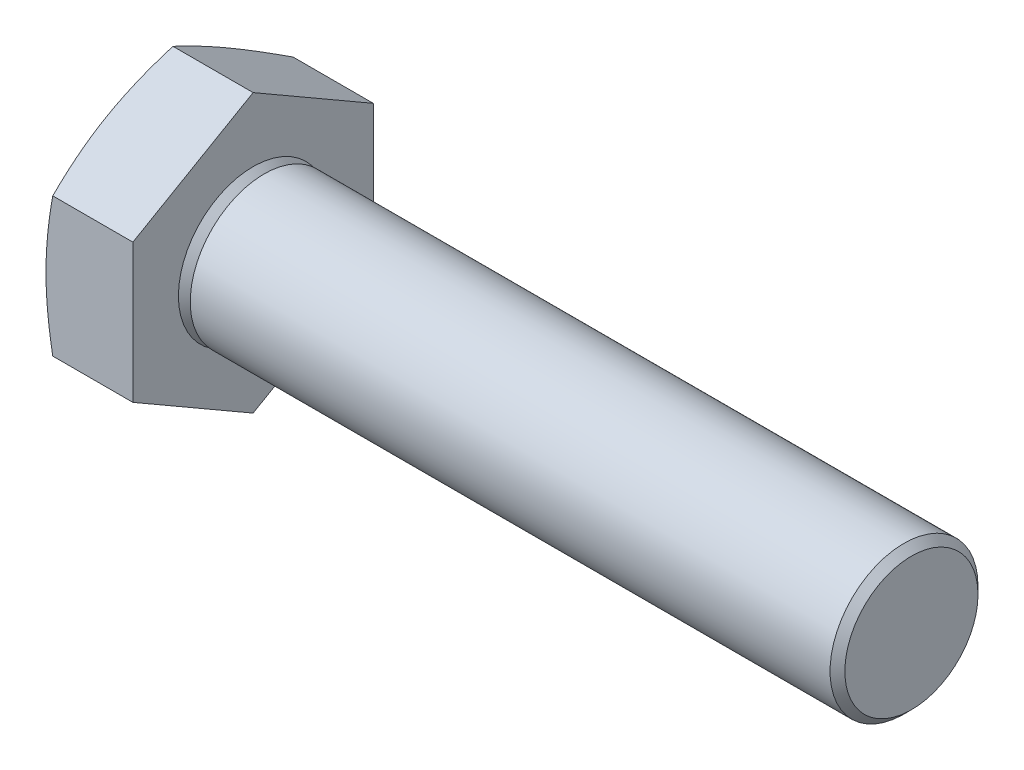
from build123d import *

# Parameters (mm, degrees)
BASEHEAD_DEPTH = 5.3
SKETCH5_R      = 4
BASEBODY_DEPTH = 35
CHAMFER1_SIZE  = 0.4


with BuildPart() as part:
    # Sketch2 → BaseHead (new body)
    with BuildSketch(Plane(origin=(0, 0, 0), x_dir=(0, 0, -1), z_dir=(1, 0, 0))):
        Polygon((6.5, -3.75277675), (6.5, 3.75277675), (0, 7.505553499), (-6.5, 3.75277675), (-6.5, -3.75277675), (0, -7.505553499), align=None)
    extrude(amount=BASEHEAD_DEPTH)

    # Sketch3 → BearingFace (revolve, cut)
    with BuildSketch(Plane.XY, mode=Mode.PRIVATE) as bearingface_sk:
        Polygon((5.3, 7.505553499), (5.3, 3.44), (4.7, 4.04), (4.7, 7.505553499), align=None)
    revolve(bearingface_sk.sketch.rotate(Axis((-0.957090588, 0, 0), (1, 0, 0)), 90), axis=Axis((-0.957090588, 0, 0), (1, 0, 0)), mode=Mode.SUBTRACT)

    # Sketch4 → HeadChamfer (revolve, cut)
    with BuildSketch(Plane.XY):
        Polygon((0, 7.505553499), (0.365991543, 7.505553499), (0, 6.5), align=None)
    revolve(axis=Axis((-0.493528746, 0, 0), (1, 0, 0)), mode=Mode.SUBTRACT)

    # Sketch5 → BaseBody (add)
    with BuildSketch(Plane(origin=(5.3, 0, 0), x_dir=(0, 0, -1), z_dir=(1, 0, 0))):
        Circle(SKETCH5_R)
    extrude(amount=BASEBODY_DEPTH)

    # Chamfer1
    chamfer1_edges = [part.edges().sort_by_distance(p)[0] for p in [
        (40.3, 0, 4),
    ]]
    chamfer(chamfer1_edges, length=CHAMFER1_SIZE)


solid = part.part
